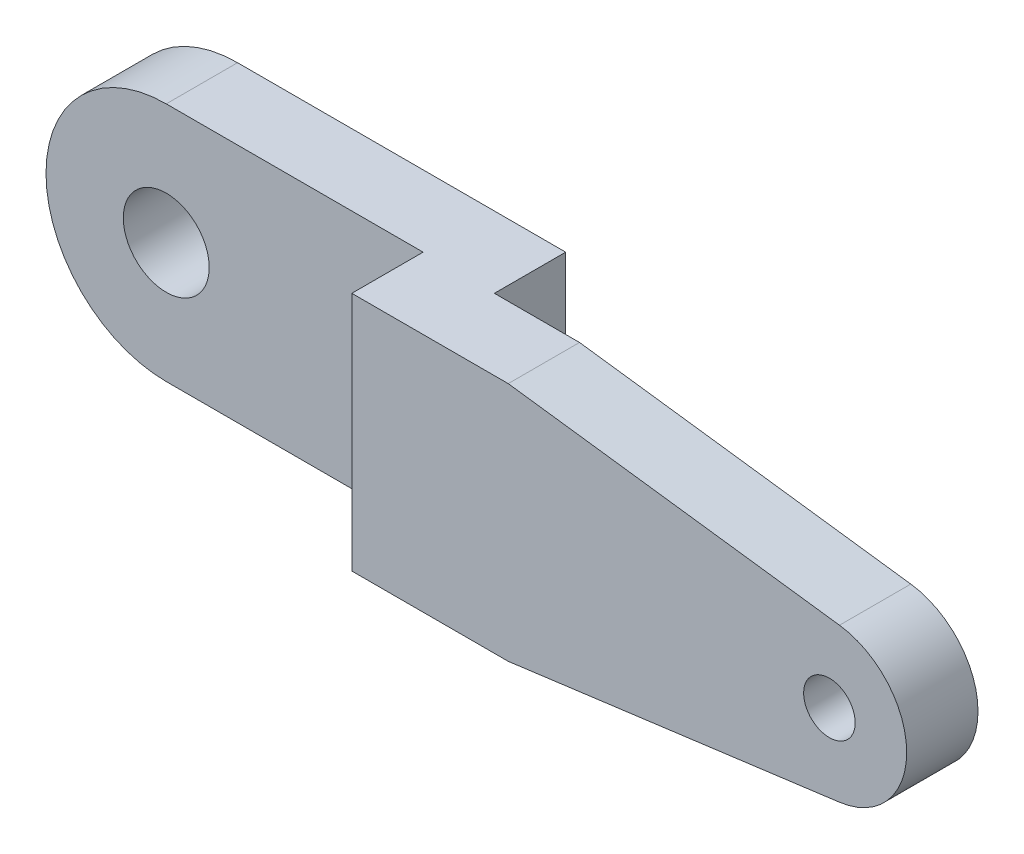
SolidWorks part; units mm, degrees
ref_plane "Front Plane" through (0, 0, 0) normal (0, 0, 1) x (1, 0, 0)
ref_plane "Top Plane" through (0, 0, 0) normal (0, 1, 0) x (1, 0, 0)
ref_plane "Right Plane" through (0, 0, 0) normal (1, 0, 0) x (0, 0, -1)
sketch "Sketch1" plane through (0, 0, 0) normal (0, 0, 1) x (1, 0, 0)
  line L0 (-43.9, 0) -> (-43.9, -19.3369) construction
  line L1 (-29.9, 14) -> (0, 14)
  line L2 (-29.9, -14) -> (0, -14)
  line L3 (0, -14) -> (0, 14)
  line L5 (0, 14) -> (8.3, 14)
  line L6 (0, 14) -> (0, -14)
  line L7 (0, -14) -> (8.3, -14)
  line L8 (8.3, 14) -> (8.3, -14)
  arc A0 (-29.9, 14) -> (-29.9, -14) centre (-29.9, 0) ccw
  circle A1 centre (-29.9, 0) radius 5
  point P10 (0, 0)
  dimension "D1" = 28
  dimension "D2" = 43.9
  dimension "D3" = 10
  dimension "D4" = 8.3
extrude "Boss-Extrude2" add sketch "Sketch1" along normal blind 8.3 contours L1 A0 L2 L3 A1 | L8 L5 L3 L7
sketch "Sketch2" plane through (0, 0, 8.3) normal (0, 0, 1) x (1, 0, 0)
  line L0 (0, 14) -> (0, -14)
  line L1 (-29.9, 14) -> (8.3, 14) construction
  line L2 (-29.9, -14) -> (8.3, -14) construction
  line L3 (0, 14) -> (18.2111, 14)
  line L4 (0, -14) -> (18.2111, -14)
  line L5 (18.2111, -14) -> (56.7747, -8.923)
  line L6 (18.2111, 14) -> (56.7747, 8.923)
  line L7 (55.6, 0) -> (20.017, 0) construction
  arc A0 (56.7747, -8.923) -> (56.7747, 8.923) centre (55.6, 0) ccw
  circle A1 centre (-29.9, 0) radius 5 construction
  circle A2 centre (55.6, 0) radius 3
  dimension "D1" = 18
  dimension "D4" = 6
  dimension "D2" = 85.5
  dimension "D3" = 15
extrude "Boss-Extrude4" add sketch "Sketch2" along normal blind 8.3
